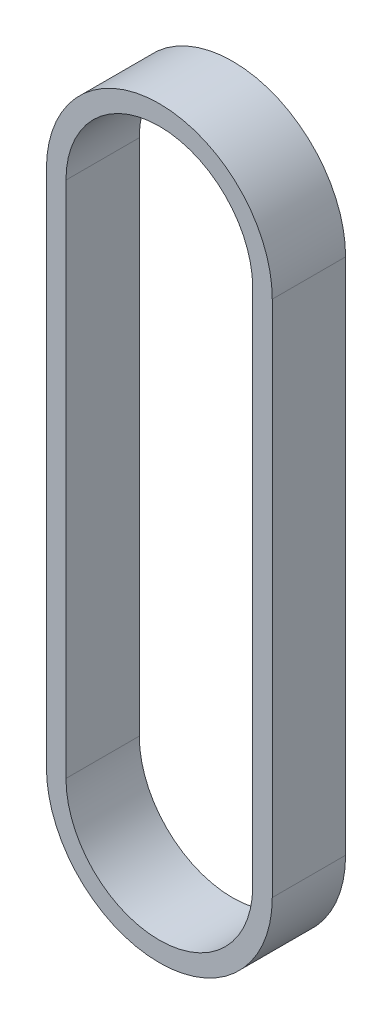
SolidWorks part; units mm, degrees
material "标准件"
ref_plane "前视基准面" through (0, 0, 0) normal (0, 0, 1) x (1, 0, 0)
ref_plane "上视基准面" through (0, 0, 0) normal (0, 1, 0) x (1, 0, 0)
ref_plane "右视基准面" through (0, 0, 0) normal (1, 0, 0) x (0, 0, -1)
sketch "草图2" plane through (0, 0, 0) normal (0, 0, 1) x (1, 0, 0)
  line L0 (0, 0) -> (1, 0) construction
  line L1 (0, 0) -> (0, 1) construction
  line L2 (-21.1, 0) -> (-21.1, 106)
  line L3 (21.1, 106) -> (21.1, 0)
  arc A0 (21.1, 0) -> (-21.1, 0) centre (0, 0) cw
  arc A1 (-21.1, 106) -> (21.1, 106) centre (0, 106) cw
extrude "拉伸-薄壁1" add sketch "草图2" along normal mid plane 15 thin thin type mid plane wall 4
